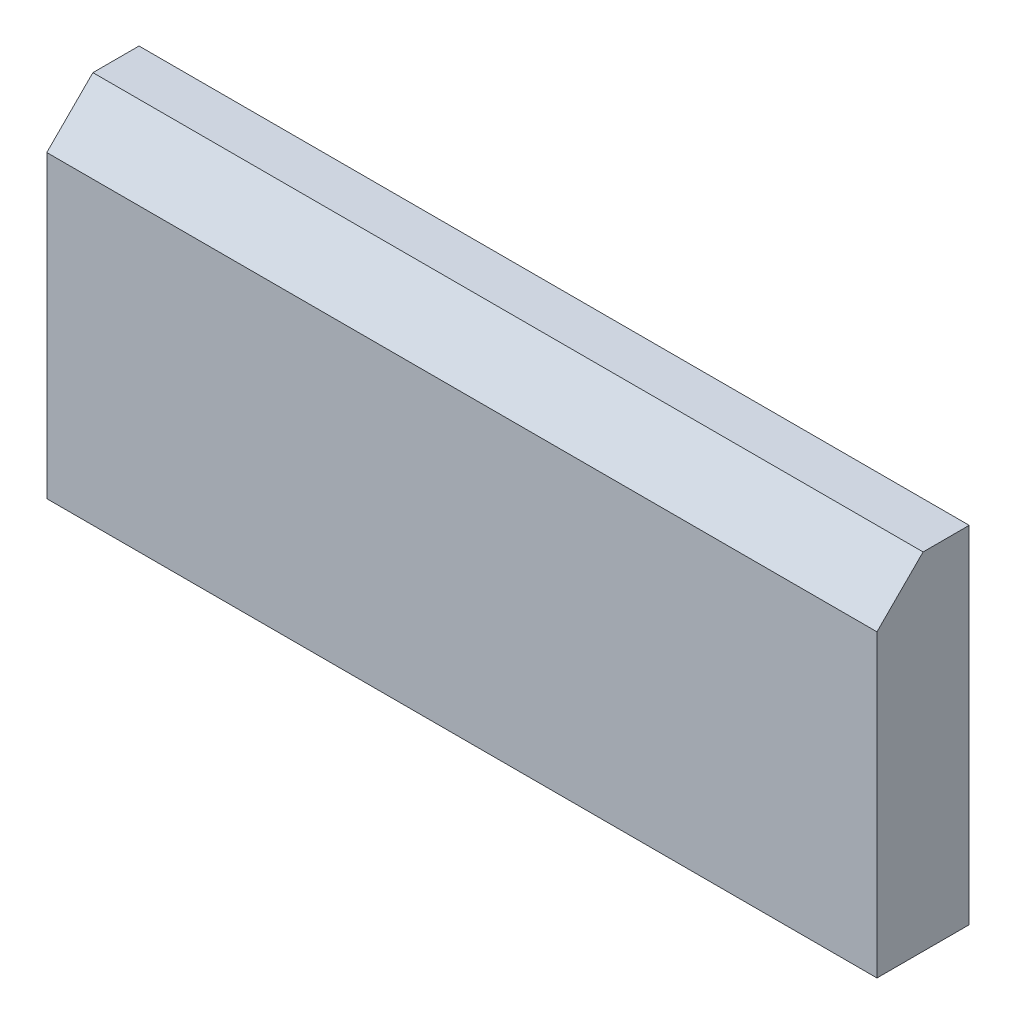
from build123d import *

# Parameters (mm, degrees)
SKETCH_1_W      = 180
SKETCH_1_H      = 75
EXTRUDE_1_DEPTH = 20
CHAMFER_2_SIZE  = 10


with BuildPart() as part:
    # 草图1 → 凸台-拉伸1 (new body)
    with BuildSketch(Plane.XY):
        with Locations((0, 37.5)):
            Rectangle(SKETCH_1_W, SKETCH_1_H)
    extrude(amount=EXTRUDE_1_DEPTH)

    # 倒角2
    chamfer_2_edges = [part.edges().sort_by_distance(p)[0] for p in [
        (0, 75, 20),
    ]]
    chamfer(chamfer_2_edges, length=CHAMFER_2_SIZE)


solid = part.part
